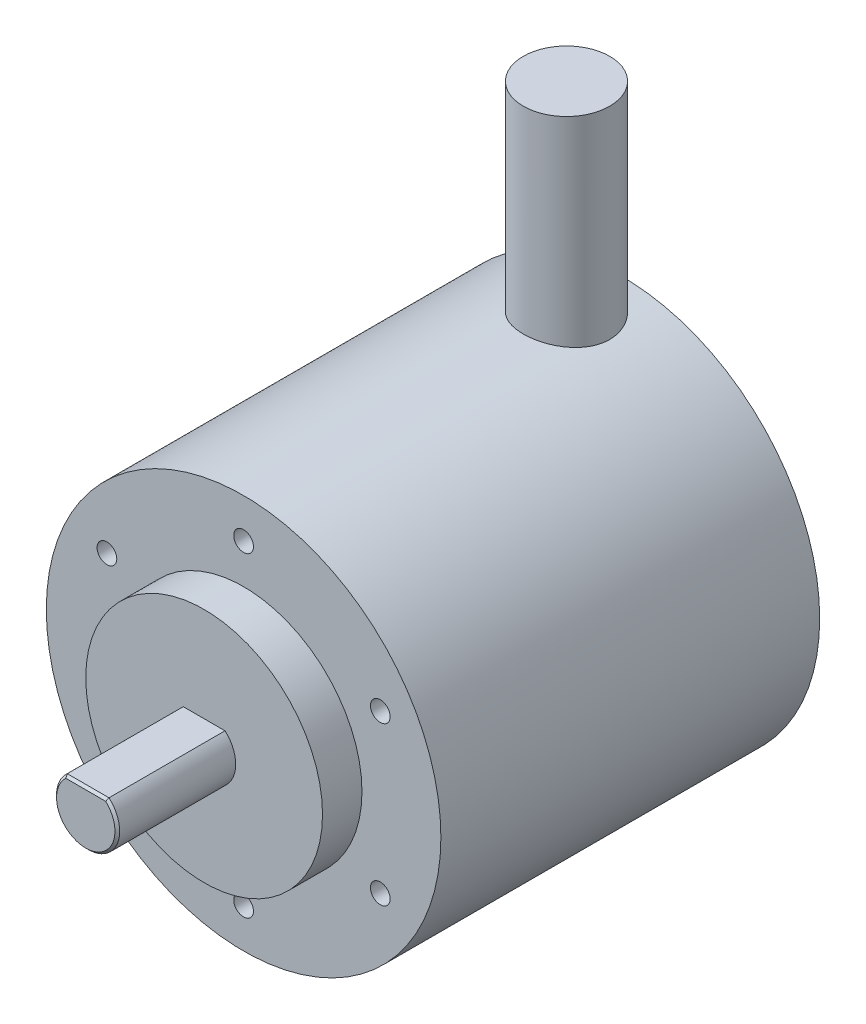
SolidWorks part; units mm, degrees
ref_plane "Front Plane" through (0, 0, 0) normal (0, 0, 1) x (1, 0, 0)
ref_plane "Top Plane" through (0, 0, 0) normal (0, 1, 0) x (1, 0, 0)
ref_plane "Right Plane" through (0, 0, 0) normal (1, 0, 0) x (0, 0, -1)
sketch "Sketch1" plane through (0, 0, 0) normal (0, 0, 1) x (1, 0, 0)
  circle A0 centre (0, 0) radius 25
  dimension "D1" = 50
extrude "Boss-Extrude1" add sketch "Sketch1" along normal blind 48
sketch "Sketch2" plane through (0, 0, 48) normal (0, 0, 1) x (1, 0, 0)
  circle A0 centre (0, 0) radius 15
  dimension "D1" = 30
extrude "Boss-Extrude2" add sketch "Sketch2" along normal blind 5
sketch "Sketch3" plane through (0, 0, 53) normal (0, 0, 1) x (1, 0, 0)
  line L0 (-2.6458, 3) -> (2.6458, 3)
  arc A0 (-2.6458, 3) -> (2.6458, 3) centre (0, 0) ccw
  dimension "D1" = 8
  dimension "D2" = 3
extrude "Boss-Extrude3" add sketch "Sketch3" along normal blind 15
chamfer "Chamfer1" distance 0.3 angle 45 2 edges at (0, 3, 68) (0, -4, 68)
sketch "Sketch4" plane through (0, 0, 0) normal (0, 1, 0) x (1, 0, 0)
  circle A0 centre (0, -7.0835) radius 5.478
extrude "Boss-Extrude4" add sketch "Sketch4" along normal blind 50
sketch "Sketch5" plane through (0, 0, 48) normal (0, 0, 1) x (1, 0, 0)
  circle A0 centre (0, 0) radius 20 construction
  circle A1 centre (0, 20) radius 1.25
  circle A2 centre (17.3205, 10) radius 1.25
  circle A3 centre (17.3205, -10) radius 1.25
  circle A4 centre (0, -20) radius 1.25
  circle A5 centre (-17.3205, -10) radius 1.25
  circle A6 centre (-17.3205, 10) radius 1.25
  point P18 (0, 0)
  dimension "D1" = 40
  dimension "D2" = 2.5
  dimension "D3" = 6
extrude "Cut-Extrude1" cut sketch "Sketch5" against normal blind 7
